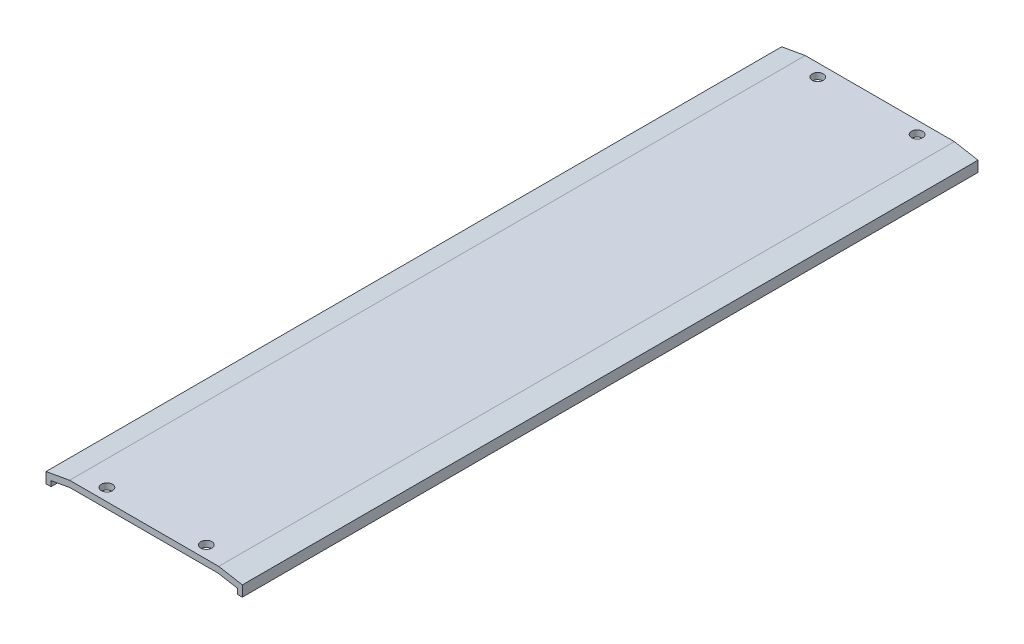
from build123d import *

# Parameters (mm, degrees)
EXTRUDE_1_DEPTH     = 148
SKETCH_2_R          = 2.25
CUT_EXTRUDE_1_DEPTH = 10


with BuildPart() as part:
    # 草图1 → 凸台-拉伸1 (new, symmetric)
    with BuildSketch(Plane.XY):
        Polygon((-37.5, 0), (-39.5, 0), (-39.5, 4.3), (-30, 6), (30, 6), (39.5, 4.3), (39.5, 0), (37.5, 0), (37.5, 2.122105263), (29.8, 3.5), (-29.8, 3.5), (-37.5, 2.122105263), align=None)
    extrude(amount=EXTRUDE_1_DEPTH, both=True)

    # 草图2 → 切除-拉伸1 (cut)
    with BuildSketch(Plane(origin=(0, 6, 0), x_dir=(1, 0, 0), z_dir=(0, 1, 0))):
        with Locations(Location((-20, -143, 0), (0, 0, 270))):
            Circle(SKETCH_2_R)
        with Locations(Location((20, -143, 0), (0, 0, 270))):
            Circle(SKETCH_2_R)
    cut_extrude_1 = extrude(amount=-CUT_EXTRUDE_1_DEPTH, mode=Mode.SUBTRACT)

    # 镜向1: 切除-拉伸1 across plane
    add(cut_extrude_1.mirror(Plane.XY), mode=Mode.SUBTRACT)


solid = part.part
